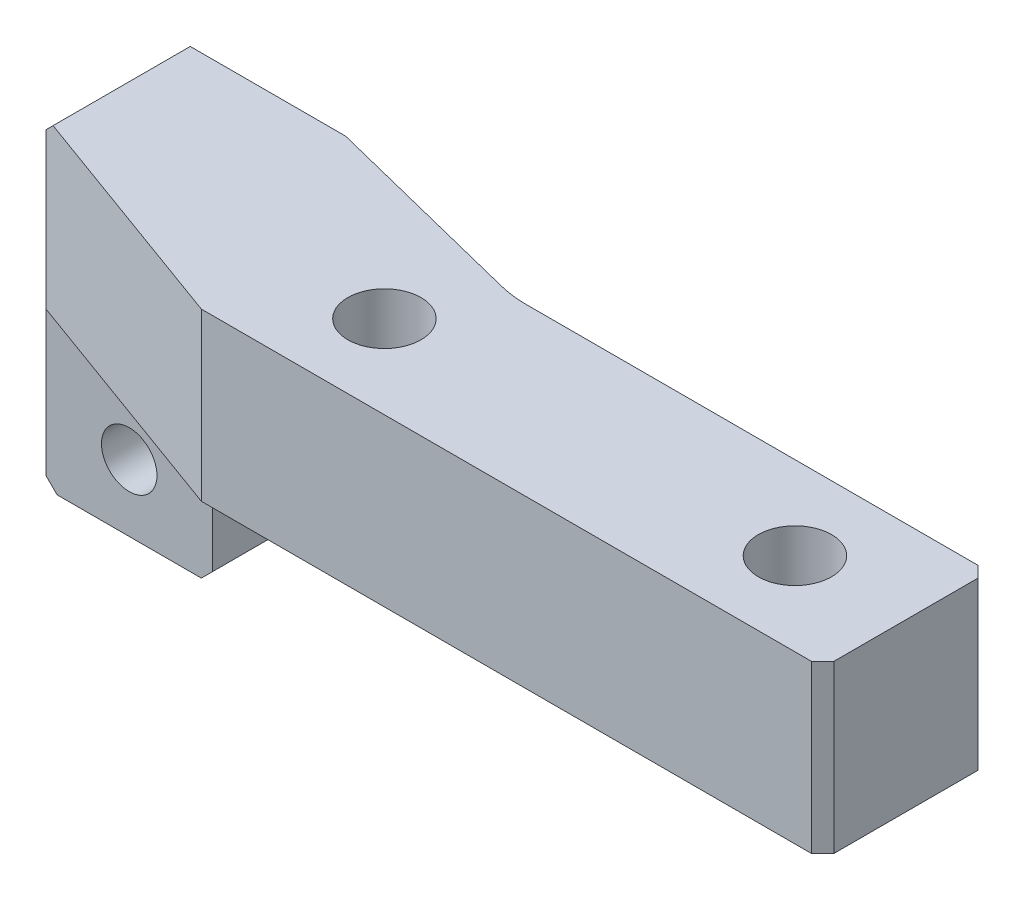
SolidWorks part; units mm, degrees
material "45#"
ref_plane "前基準面" through (0, 0, 0) normal (0, 0, 1) x (1, 0, 0)
ref_plane "上基準面" through (0, 0, 0) normal (0, 1, 0) x (1, 0, 0)
ref_plane "右基準面" through (0, 0, 0) normal (1, 0, 0) x (0, 0, -1)
sketch "草图1" plane through (0, 0, 0) normal (0, 1, 0) x (1, 0, 0)
  line L1 (-39, -7.5) -> (39, -7.5)
  line L2 (-39, -7.5) -> (-39, 7.5)
  line L3 (-39, 7.5) -> (39, 7.5)
  line L4 (39, -7.5) -> (39, 7.5)
  line L5 (-39, -7.5) -> (39, 7.5) construction
  line L6 (-39, 7.5) -> (39, -7.5) construction
  point P0 (0, 0)
  dimension "D1" = 78
  dimension "D2" = 15
extrude "凸台-拉伸1" add sketch "草图1" along normal mid plane 15
sketch "草图3" plane through (0, -7.5, 0) normal (0, 1, 0) x (1, 0, 0)
  line L0 (39, -7.5) -> (39, 7.5) construction
  point P0 (29, 0)
  point P2 (-8, 0)
  dimension "D1" = 37
  dimension "D2" = 10
hole_wizard "M6 六角圆柱头螺钉的柱形沉头孔1" positions "草图3" profile "草图4" counterbore size "M6" standard "GB" end condition through all
sketch "草图4" plane through (29, -7.5, 0) normal (1, 0, 0) x (0, 0, -1)
  line L0 (0, 0) -> (0, 15)
  line L1 (0, 15) -> (3.3, 15)
  line L3 (3.3, 15) -> (3.3, 6.8)
  line L4 (3.3, 6.8) -> (5.5, 6.8)
  line L5 (5.5, 6.8) -> (5.5, 0)
  line L7 (5.5, 0) -> (0, 0)
  line L11 (0, -6.35) -> (0, 107.95) construction
  dimension "通孔孔直径" = 6.6
  dimension "通孔孔深度" = 15
  dimension "柱形沉头孔直径" = 11
  dimension "柱形沉头孔深度" = 6.8
sketch "草图8" plane through (0, 7.5, 0) normal (0, 1, 0) x (1, 0, 0)
  line L0 (-8, 0) -> (29, 0) construction
  line L2 (-24, 12.5) -> (-39, 12.5)
  line L3 (-39, 12.5) -> (-39, 7.5)
  line L4 (-39, 7.5) -> (-4, 7.5)
  line L5 (10.5, 0) -> (10.5, 27.5008) construction
  line L6 (39, 7.5) -> (-39, 7.5) construction
  line L7 (-4, 7.5) -> (-24, 12.5)
  line L8 (-39, -7.5) -> (39, -7.5) construction
  dimension "D2" = 15
  dimension "D1" = 35
  dimension "D3" = 20
extrude "凸台-拉伸3" add sketch "草图8" against normal up to surface (15 mm away) up to face at (29, -7.5, -5.5)
sketch "草图2" plane through (0, -7.5, 0) normal (0, 1, 0) x (1, 0, 0)
  line L1 (-39, 12.5) -> (-24, 12.5)
  line L2 (-39, 12.5) -> (-39, 0.5)
  line L3 (-39, 0.5) -> (-24, 0.5)
  line L4 (-24, 12.5) -> (-24, 0.5)
  line L5 (-39, 12.5) -> (-39, -7.5) construction
  line L6 (-24, 12.5) -> (-39, 12.5) construction
  dimension "D1" = 15
  dimension "D2" = 12
extrude "凸台-拉伸2" add sketch "草图2" against normal blind 14
sketch "草图5" plane through (-28.5, 0, -0.5) normal (0, 0, 1) x (1, 0, 0)
  line L2 (-3, -21.5) -> (-3, 18.3388) construction
  line L5 (-10.5, -21.5) -> (4.5, -21.5) construction
  point P0 (-3, -15.5)
  dimension "D1" = 6
hole_wizard "M6 螺纹孔1" positions "草图5" profile "草图6" tap size "M6" standard "GB" end condition through all
sketch "草图6" plane through (-31.5, -15.5, -0.5) normal (1, 0, 0) x (0, -1, 0)
  line L0 (0, 0) -> (0, 12)
  line L1 (0, 12) -> (2.5, 12)
  line L2 (2.5, 12) -> (2.5, 0)
  line L5 (2.5, 0) -> (0, 0)
  line L11 (0, -6.35) -> (0, 107.95) construction
  dimension "通孔螺纹孔钻头直径" = 5
  dimension "通孔螺纹孔钻头深度" = 12
cosmetic thread "孔螺纹线1" parameters "D2"=6
sketch "草图9" plane through (0, -21.5, 0) normal (0, -1, 0) x (-1, 0, 0)
  line L0 (39, -7.5) -> (-39, -7.5) construction
  line L2 (39, 0.5) -> (39, -7.5)
  line L3 (39, -7.5) -> (17, -7.5)
  line L6 (39, 0.5) -> (17, -7.5)
  line L7 (39, -7.5) -> (-39, -7.5) construction
  dimension "D1" = 22
extrude "切除-拉伸1" cut sketch "草图9" against normal through all
chamfer "倒角1" distance 1 angle 45 5 edges at (39, 0, -7.5) (39, 0, 7.5) (-39, -21.5, -6.5) (-24, -21.5, -6.5) (-39, 7.5, -6.5)
fillet "圆角2" radius 10 1 edges at (-4, 0, -7.5)
